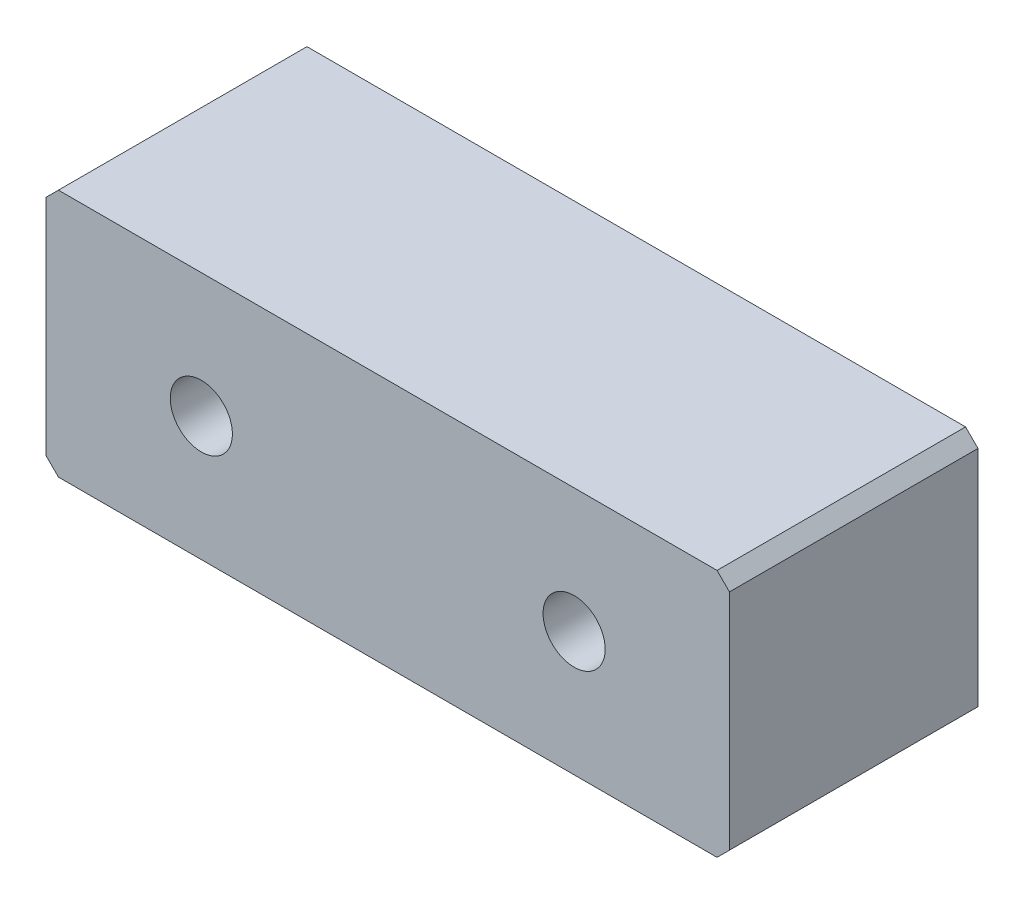
SolidWorks part; units mm, degrees
ref_plane "Front Plane" through (0, 0, 0) normal (0, 0, 1) x (1, 0, 0)
ref_plane "Top Plane" through (0, 0, 0) normal (0, 1, 0) x (1, 0, 0)
ref_plane "Right Plane" through (0, 0, 0) normal (1, 0, 0) x (0, 0, -1)
sketch "Sketch1" plane through (0, 0, 0) normal (0, 0, 1) x (1, 0, 0)
  line L1 (-79.8363, 38.0556) -> (-24.8363, 38.0556)
  line L2 (-79.8363, 38.0556) -> (-79.8363, 18.0556)
  line L3 (-79.8363, 18.0556) -> (-24.8363, 18.0556)
  line L4 (-24.8363, 38.0556) -> (-24.8363, 18.0556)
  dimension "D1" = 55
  dimension "D2" = 20
extrude "Boss-Extrude1" add sketch "Sketch1" along normal blind 20
sketch "Sketch2" plane through (0, 0, 20) normal (0, 0, 1) x (1, 0, 0)
  line L0 (-67.3363, 28.0556) -> (-37.3363, 28.0556)
  line L1 (-24.8363, 18.0556) -> (-24.8363, 38.0556) construction
  line L2 (-79.8363, 18.0556) -> (-24.8363, 18.0556) construction
  dimension "D1" = 30
  dimension "D2" = 12.5
  dimension "D3" = 10
hole_wizard "M6 Tapped Hole1" positions "Sketch3" profile "Sketch4" tap size "M6" standard "GB" end condition through all
sketch "Sketch3" plane through (0, 0, 20) normal (0, 0, 1) x (1, 0, 0)
  point P0 (-67.3363, 28.0556)
  point P3 (-37.3363, 28.0556)
sketch "Sketch4" plane through (-67.3363, 28.0556, 20) normal (1, 0, 0) x (0, -1, 0)
  line L0 (0, 0) -> (0, 20)
  line L1 (0, 20) -> (2.5, 20)
  line L2 (2.5, 20) -> (2.5, 0)
  line L5 (2.5, 0) -> (0, 0)
  line L11 (0, -6.35) -> (0, 107.95) construction
  dimension "通孔螺纹孔钻头直径" = 5
  dimension "通孔螺纹孔钻头深度" = 20
cosmetic thread "Cosmetic thread 1" parameters "D2"=6
cosmetic thread "Cosmetic thread 2" parameters "D2"=6
chamfer "Chamfer1" distance 1 angle 45 4 edges at (-24.8363, 38.0556, 10) (-24.8363, 18.0556, 10) (-79.8363, 18.0556, 10) (-79.8363, 38.0556, 10)
